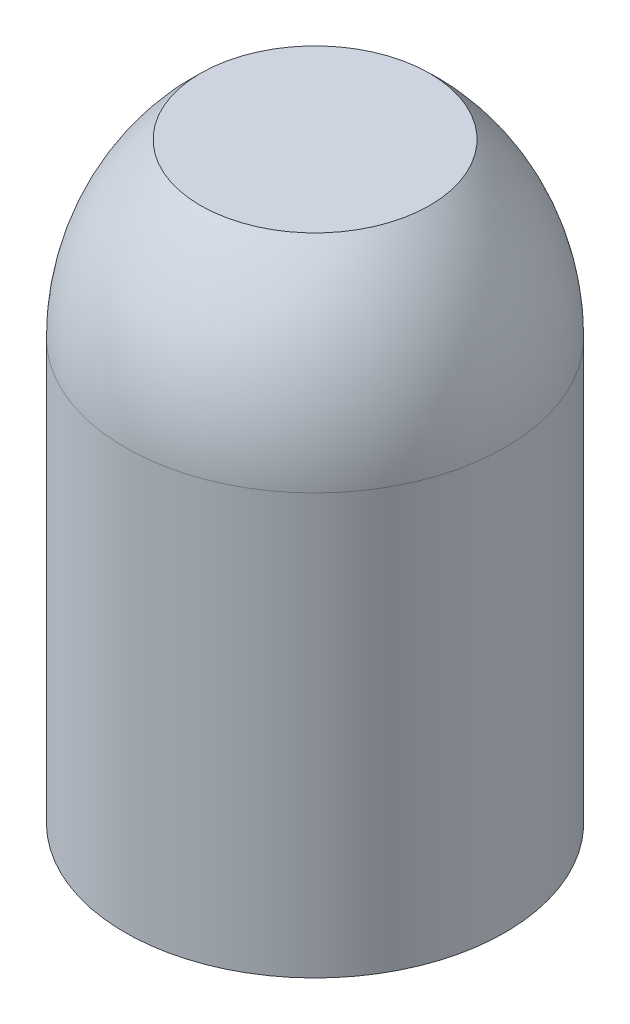
from build123d import *

# Parameters (mm, degrees)
M3_TAPPED_HOLE1_D     = 2.5
M3_TAPPED_HOLE1_DEPTH = 7.5
M3_TAPPED_HOLE1_TIP   = 0.751075774


with BuildPart() as part:
    # Sketch1 → Revolve1 (revolve)
    with BuildSketch(Plane.XY, mode=Mode.PRIVATE) as revolve1_sk:
        with BuildLine():
            Line((0, 0), (-4.975, 0))
            Line((-4.975, 0), (-4.975, 11))
            ThreePointArc((-4.975, 11), (-4.459519856, 13.45716427), (-3, 15.5))
            Line((-3, 15.5), (0, 15.5))
            Line((0, 15.5), (0, 0))
        make_face()
    revolve(revolve1_sk.sketch.rotate(Axis((0, 0, 0), (0, 1, 0)), 270), axis=Axis((0, 0, 0), (0, 1, 0)))

    # M3 Tapped Hole1
    with Locations(Plane(origin=(0, 0, 0), x_dir=(-1, 0, 0), z_dir=(0, -1, 0))):
        with Locations((0, 0)):
            Hole(M3_TAPPED_HOLE1_D / 2, depth=M3_TAPPED_HOLE1_DEPTH)
            with Locations((0, 0, -(M3_TAPPED_HOLE1_DEPTH + M3_TAPPED_HOLE1_TIP / 2))):  # 118° drill point
                Cone(0, M3_TAPPED_HOLE1_D / 2, M3_TAPPED_HOLE1_TIP, mode=Mode.SUBTRACT)


solid = part.part
